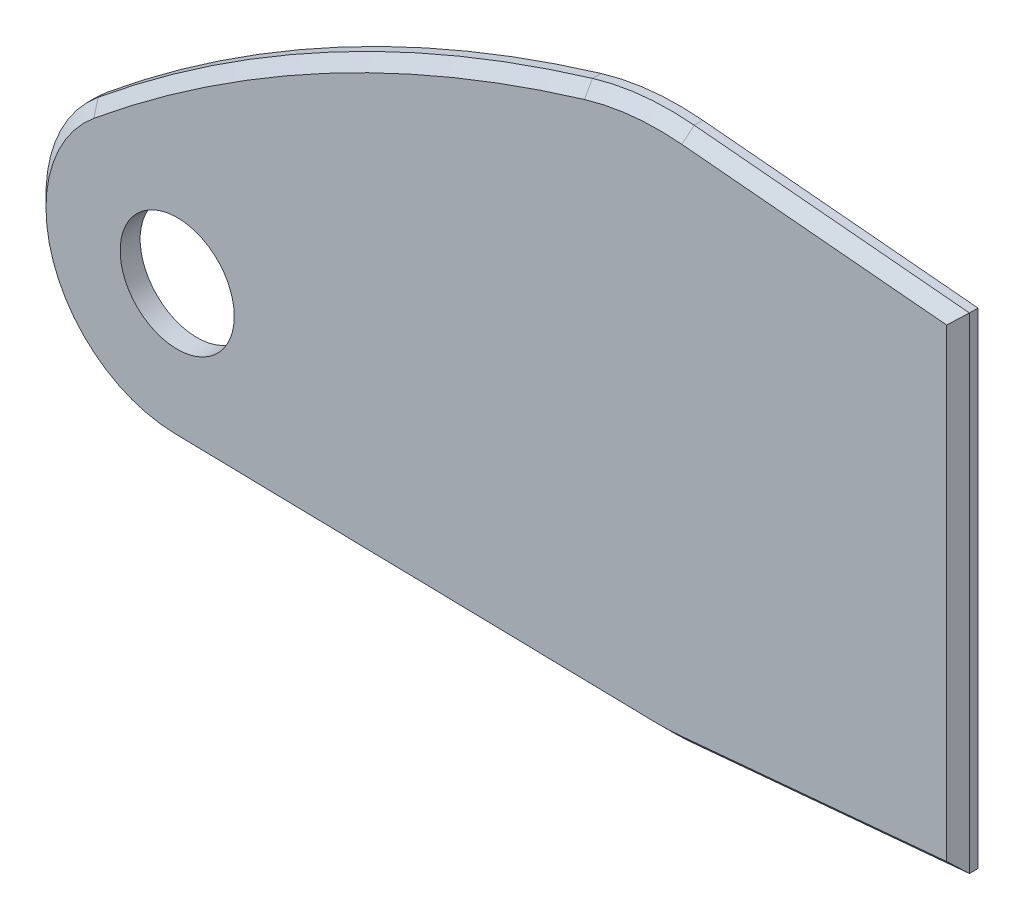
from build123d import *

# Parameters (mm, degrees)
SKETCH1_R           = 40
BOSS_EXTRUDE1_DEPTH = 14
CHAMFER1_SIZE       = 8


with BuildPart() as part:
    # Sketch1 → Boss-Extrude1 (new body)
    with BuildSketch(Plane.XY):
        with BuildLine():
            Line((210, 170.2), (17.052877352, 187.727060846))
            ThreePointArc((17.052877352, 187.727060846), (-18.959205139, 187.54412425), (-54.27928922, 180.515951544))
            ThreePointArc((-54.27928922, 180.515951544), (-236.788094268, 105.291584642), (-400.963833305, -4.319071808))
            ThreePointArc((-400.963833305, -4.319071808), (-431.989523554, -114.33728667), (-339.549522969, -181.578995072))
            Line((-339.549522969, -181.578995072), (-3.863350797, -188.460405711))
            ThreePointArc((-3.863350797, -188.460405711), (6.604949005, -188.384247347), (17.052877352, -187.727060846))
            Line((17.052877352, -187.727060846), (210, -170.2))
            Line((210, -170.2), (210, 170.2))
        make_face()
        with Locations((-337.5, -81.6)):
            Circle(SKETCH1_R, mode=Mode.SUBTRACT)
    extrude(amount=BOSS_EXTRUDE1_DEPTH)

    # Chamfer1
    chamfer1_edges = [part.edges().sort_by_distance(p)[0] for p in [
        (6.604949005, -188.384247347, 14),
        (113.526438676, -178.963530423, 14),
        (210, 0, 14),
        (113.526438676, 178.963530423, 14),
        (-18.959205139, 187.54412425, 14),
        (-236.788094268, 105.291584642, 14),
        (-431.989523554, -114.33728667, 14),
        (-171.706436883, -185.019700391, 14),
    ]]
    chamfer(chamfer1_edges, length=CHAMFER1_SIZE)


solid = part.part
